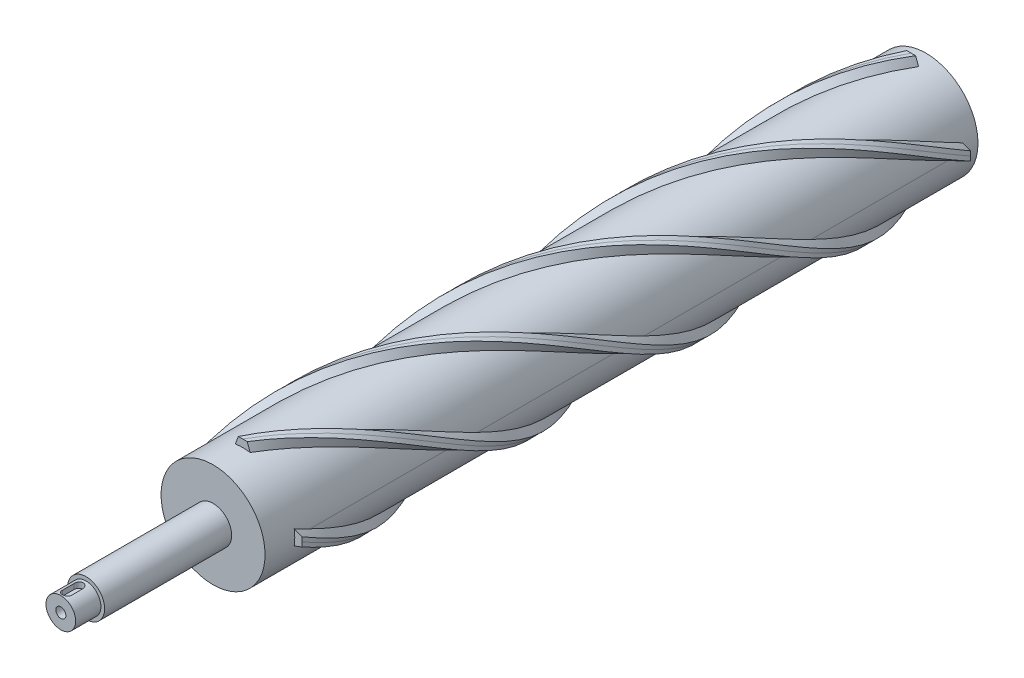
SolidWorks part; units mm, degrees
ref_plane "前视基准面" through (0, 0, 0) normal (0, 0, 1) x (1, 0, 0)
ref_plane "上视基准面" through (0, 0, 0) normal (0, 1, 0) x (1, 0, 0)
ref_plane "右视基准面" through (0, 0, 0) normal (1, 0, 0) x (0, 0, -1)
sketch "草图1" plane through (0, 0, 0) normal (0, 0, 1) x (1, 0, 0)
  circle A0 centre (0, 0) radius 15
extrude "凸台-拉伸1" add sketch "草图1" along normal blind 10
sketch "草图2" plane through (0, 0, 10) normal (0, 0, 1) x (1, 0, 0)
  circle A0 centre (0, 0) radius 35
extrude "凸台-拉伸2" add sketch "草图2" along normal blind 480
sketch "草图3" plane through (0, 0, 490) normal (0, 0, 1) x (1, 0, 0)
  circle A0 centre (0, 0) radius 12.5
extrude "凸台-拉伸3" add sketch "草图3" along normal blind 85.5
ref_plane "基准面1" through (0, 0, 20) normal (0, 0, -1) x (-1, 0, 0)
sketch "草图4" plane through (0, 0, 20) normal (0, 0, -1) x (-1, 0, 0)
  circle A0 centre (0, 0) radius 35
curve "螺旋线/涡状线1" pitch 450 height 450 turns 1
sketch "草图6" plane through (0, 0, 20) normal (0, 0, -1) x (-1, 0, 0)
  line L0 (0, 0) -> (0, 43.7073) construction
  line L1 (-5, 34.641) -> (-5, 32.641)
  line L2 (0, 40) -> (3, 40)
  line L3 (-5, 32.641) -> (5, 32.641)
  line L4 (5, 32.641) -> (5, 34.641)
  line L5 (-3, 40) -> (-5, 34.641)
  line L6 (0, 40) -> (-3, 40)
  line L7 (34.641, 5) -> (32.641, 5)
  line L8 (40, 0) -> (40, -3)
  line L9 (32.641, 5) -> (32.641, -5)
  line L10 (3, 40) -> (5, 34.641)
  line L11 (32.641, -5) -> (34.641, -5)
  line L12 (40, 3) -> (34.641, 5)
  line L13 (40, 0) -> (40, 3)
  line L14 (40, -3) -> (34.641, -5)
  line L15 (5, -34.641) -> (5, -32.641)
  line L16 (0, -40) -> (-3, -40)
  line L17 (5, -32.641) -> (-5, -32.641)
  line L18 (-5, -32.641) -> (-5, -34.641)
  line L19 (3, -40) -> (5, -34.641)
  line L20 (0, -40) -> (3, -40)
  line L21 (-3, -40) -> (-5, -34.641)
  line L22 (-34.641, -5) -> (-32.641, -5)
  line L23 (-40, 0) -> (-40, 3)
  line L24 (-32.641, -5) -> (-32.641, 5)
  line L25 (-32.641, 5) -> (-34.641, 5)
  line L26 (-40, -3) -> (-34.641, -5)
  line L27 (-40, 0) -> (-40, -3)
  line L28 (-40, 3) -> (-34.641, 5)
  point P34 (0, 0)
  dimension "D1" = 4
sweep "扫描1" add profiles "草图6" path "螺旋线/涡状线1"
sketch "草图7" plane through (0, 0, 575.5) normal (0, 0, 1) x (1, 0, 0)
  circle A0 centre (0, 0) radius 10
extrude "凸台-拉伸4" add sketch "草图7" along normal blind 17
ref_plane "基准面2" through (0, 10, 0) normal (0, 1, 0) x (1, 0, 0)
sketch "草图8" plane through (0, 10, 0) normal (0, 1, 0) x (1, 0, 0)
  line L0 (0, -580.5) -> (0, -588.5) construction
  line L1 (3, -580.5) -> (3, -588.5)
  line L2 (-3, -580.5) -> (-3, -588.5)
  line L3 (-10, -575.5) -> (10, -575.5) construction
  arc A0 (3, -580.5) -> (-3, -580.5) centre (0, -580.5) ccw
  arc A1 (-3, -588.5) -> (3, -588.5) centre (0, -588.5) ccw
  point P3 (0, -584.5)
  dimension "D1" = 8
  dimension "D2" = 3
  dimension "D3" = 5
extrude "切除-拉伸1" cut sketch "草图8" against normal blind 3.96
hole_wizard "M8 螺纹孔1" positions "草图10" profile "草图9" tap size "M8" standard "Iso"
sketch "草图10" plane through (0, 0, 592.5) normal (0, 0, 1) x (1, 0, 0)
  point P0 (0, 0)
sketch "草图9" plane through (0, 0, 592.5) normal (1, 0, 0) x (0, -1, 0)
  line L0 (0, 0) -> (0, 17.0429)
  line L1 (0, 17.0429) -> (3.4, 15)
  line L2 (3.4, 15) -> (3.4, 0)
  line L5 (3.4, 0) -> (0, 0)
  line L10 (0, 17.0429) -> (-3.4, 15) construction
  line L11 (0, -6.35) -> (0, 107.95) construction
  dimension "螺纹孔钻头直径" = 6.8
  dimension "螺纹孔钻头深度" = 15
  dimension "导头角度" = 118
cosmetic thread "孔螺蚊线1" parameters "D1"=15, "D2"=8
